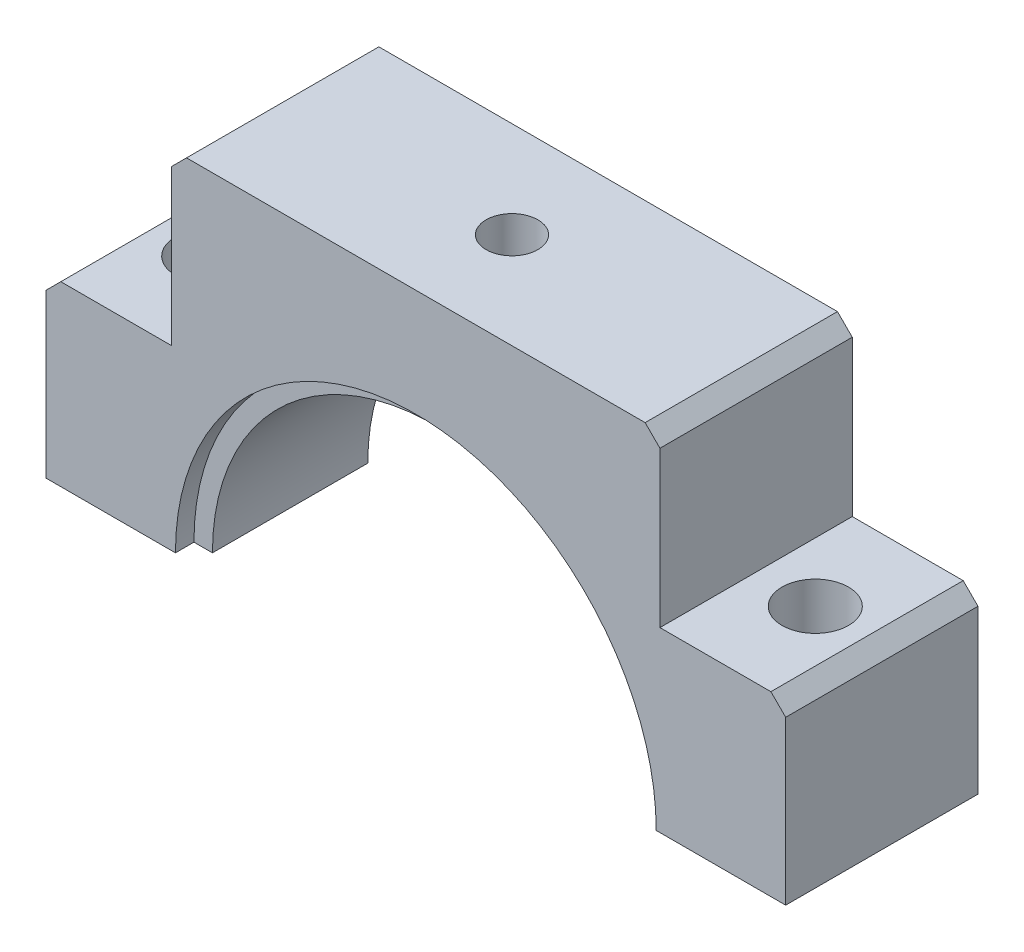
from build123d import *

# Parameters (mm, degrees)
BOSS_EXTRUDE1_DEPTH       = 26
CHAMFER1_SIZE             = 2
M8X1_0_TAPPED_HOLE1_D     = 7
M8X1_0_TAPPED_HOLE1_DEPTH = 11
M8X1_0_TAPPED_HOLE1_TIP   = 2.103012167
HOLE2_D                   = 9
SKETCH11_R                = 32.5
CUT_EXTRUDE1_DEPTH        = 2.5
CUT_EXTRUDE2_START        = -2.5
SKETCH12_R                = 32.5
CUT_EXTRUDE2_DEPTH        = 2.5
HOLE3_D                   = 4


with BuildPart() as part:
    # Sketch1 → Boss-Extrude1 (new body)
    with BuildSketch(Plane.XY):
        with BuildLine():
            Line((-50, 24), (-33, 24))
            Line((-33, 24), (-33, 47))
            Line((-33, 47), (33, 47))
            Line((33, 47), (33, 24))
            Line((33, 24), (50, 24))
            Line((50, 24), (50, 0))
            Line((50, 0), (30, 0))
            ThreePointArc((30, 0), (0, 30), (-30, 0))
            Line((-30, 0), (-50, 0))
            Line((-50, 0), (-50, 24))
        make_face()
    extrude(amount=BOSS_EXTRUDE1_DEPTH)

    # Chamfer1
    chamfer1_edges = [part.edges().sort_by_distance(p)[0] for p in [
        (-50, 24, 13),
        (-33, 47, 13),
        (33, 47, 13),
        (50, 24, 13),
    ]]
    chamfer(chamfer1_edges, length=CHAMFER1_SIZE)

    # M8x1.0 Tapped Hole1
    with Locations(Plane(origin=(0, 47, 0), x_dir=(1, 0, 0), z_dir=(0, 1, 0))):
        with Locations((0, -13)):
            Hole(M8X1_0_TAPPED_HOLE1_D / 2, depth=M8X1_0_TAPPED_HOLE1_DEPTH)
            with Locations((0, 0, -(M8X1_0_TAPPED_HOLE1_DEPTH + M8X1_0_TAPPED_HOLE1_TIP / 2))):  # 118° drill point
                Cone(0, M8X1_0_TAPPED_HOLE1_D / 2, M8X1_0_TAPPED_HOLE1_TIP, mode=Mode.SUBTRACT)

    # Hole2 (through all)
    with Locations(Plane(origin=(0, 24, 0), x_dir=(1, 0, 0), z_dir=(0, 1, 0))):
        with Locations((-41, -13), (41, -13)):
            Hole(HOLE2_D / 2)

    # Sketch11 → Cut-Extrude1 (cut)
    with BuildSketch(Plane.XY.offset(26)):
        Circle(SKETCH11_R)
    extrude(amount=-CUT_EXTRUDE1_DEPTH, mode=Mode.SUBTRACT)

    # Sketch12 → Cut-Extrude2 (cut)
    with BuildSketch(Plane(origin=(0, 0, 0), x_dir=(-1, 0, 0), z_dir=(0, 0, -1)).offset(CUT_EXTRUDE2_START)):
        Circle(SKETCH12_R)
    extrude(amount=CUT_EXTRUDE2_DEPTH, mode=Mode.SUBTRACT)

    # Hole3 (through all)
    with Locations(Plane(origin=(0, 47, 0), x_dir=(1, 0, 0), z_dir=(0, 1, 0))):
        with Locations((0, -13)):
            Hole(HOLE3_D / 2)


solid = part.part
